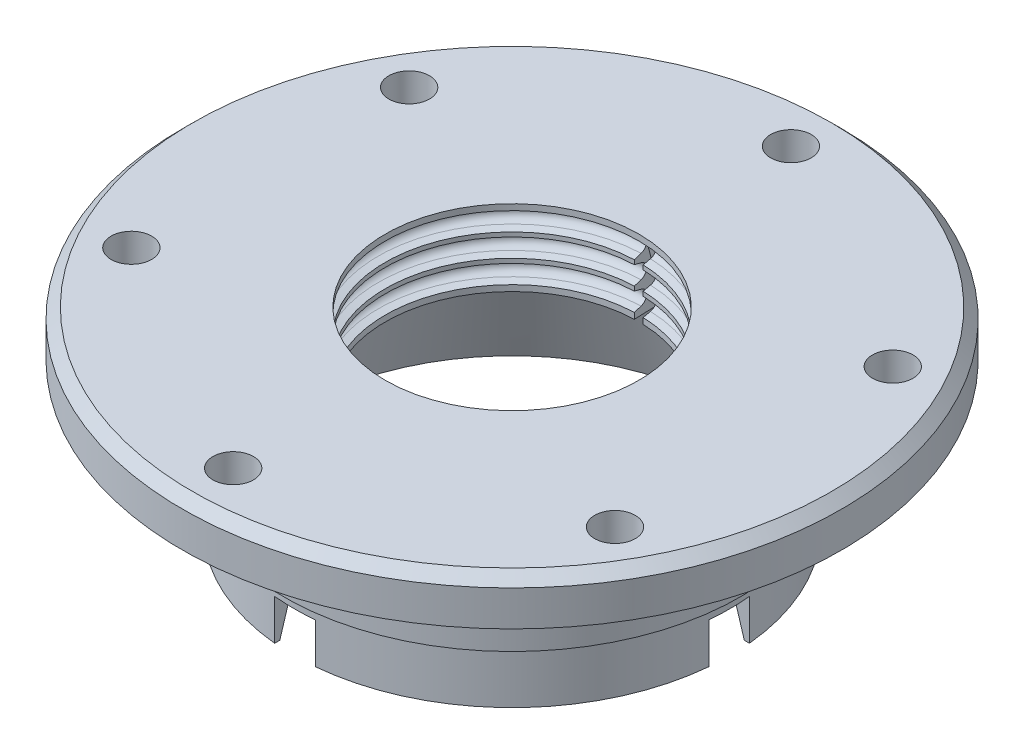
from build123d import *

# Parameters (mm, degrees)
FILLET1_R          = 5
SKETCH2_W          = 46.38448916527463
SKETCH2_H          = 8
CUT_EXTRUDE1_DEPTH = 4
SKETCH3_W          = 119.06569659747659
SKETCH3_H          = 8
CUT_EXTRUDE2_DEPTH = 4
CUT_REVOLVE2_ANGLE = 4.000000000000009
SKETCH5_R          = 3.999999999999999
SKETCH5_R_2        = 4.000000000000001
SKETCH5_R_3        = 4.000000000000005
CUT_EXTRUDE3_DEPTH = 94
SCALE_1_SCALE      = 1.875


with BuildPart() as part:
    # Sketch1 → Revolve1 (revolve)
    with BuildSketch(Plane.XY, mode=Mode.PRIVATE) as revolve1_sk:
        with BuildLine():
            Line((-43, -1.2e-16), (-43, 11))
            Line((-43, 11), (-45.00000000000001, 10.999999999999998))
            Line((-45.00000000000001, 10.999999999999998), (-45.00000000000001, 26.999999999999996))
            Line((-45.00000000000001, 26.999999999999996), (-43, 26.999999999999996))
            Line((-43, 26.999999999999996), (-43, 28.999999999999996))
            Line((-43, 28.999999999999996), (-65, 28.99999999999999))
            Line((-65, 28.99999999999999), (-65, 36))
            Line((-65, 36), (-63, 38))
            Line((-63, 38), (-25, 38))
            Line((-25, 38), (-25, 36.82086346304624))
            Line((-25, 36.82086346304624), (-26.388228567653783, 36.44888873943359))
            ThreePointArc((-26.388228567653783, 36.44888873943359), (-27.5, 34.99999999999999), (-26.388228567653783, 33.55111126056639))
            Line((-26.388228567653783, 33.55111126056639), (-25, 33.17913653695374))
            Line((-25, 33.17913653695374), (-25, 32.32086346304623))
            Line((-25, 32.32086346304623), (-26.38822856765378, 31.948888739433585))
            ThreePointArc((-26.38822856765378, 31.948888739433585), (-27.499999999999986, 30.5), (-26.388228567653783, 29.051111260566397))
            Line((-26.388228567653783, 29.051111260566397), (-25, 28.679136536953745))
            Line((-25, 28.679136536953745), (-25, 27.807055903779258))
            Line((-25, 27.807055903779258), (-26.57755901026072, 27.384350240967457))
            ThreePointArc((-26.57755901026072, 27.384350240967457), (-27.496662016431728, 25.899985958133367), (-26.38822856765378, 24.551111260566397))
            Line((-26.38822856765378, 24.551111260566397), (-25, 24.179136536953752))
            Line((-25, 24.179136536953752), (-24.999999999999996, 23))
            Line((-24.999999999999996, 23), (-34.99999999999999, 23))
            Line((-34.99999999999999, 23), (-42, 0))
            Line((-42, 0), (-43, -1.2e-16))
        make_face()
    revolve(revolve1_sk.sketch.rotate(Axis((0, 0, 0), (0, 1, 0)), 270), axis=Axis((0, 0, 0), (0, 1, 0)))

    # Fillet1
    fillet1_edges = [part.edges().sort_by_distance(p)[0] for p in [
        (-1.206e-14, 23, 34.99999999999999),
    ]]
    fillet(fillet1_edges, radius=FILLET1_R)

    # Sketch2 → Cut-Extrude1 (cut, symmetric)
    with BuildSketch(Plane.XY):
        with Locations((41.27123839114988, 4)):
            Rectangle(SKETCH2_W, SKETCH2_H)
        Polygon((-21.00085139372669, -1.2e-16), (-54.05436532646177, -1.2e-16), (-54.05436532646177, 7.9999999999999964), (-21.00085139372669, 8), align=None)
    extrude(amount=CUT_EXTRUDE1_DEPTH, both=True, mode=Mode.SUBTRACT)

    # Sketch3 → Cut-Extrude2 (cut, symmetric)
    with BuildSketch(Plane(origin=(0, 0, 0), x_dir=(0, 0, -1), z_dir=(1, 0, 0))):
        with Locations((-3.469705882441801, 4)):
            Rectangle(SKETCH3_W, SKETCH3_H)
    extrude(amount=CUT_EXTRUDE2_DEPTH, both=True, mode=Mode.SUBTRACT)

    # Sketch4 → Cut-Revolve2 (revolve, symmetric, cut)
    with BuildSketch(Plane(origin=(0, 0, 0), x_dir=(0, 0, -1), z_dir=(1, 0, 0))) as cut_revolve2_sk:
        with BuildLine():
            Line((-27.4488887394336, 35.38822856765377), (-30.768304579788595, 23))
            Line((-30.768304579788595, 23), (-24.499999999999996, 23))
            Line((-24.499999999999996, 23), (-24.499999999999996, 34.99999999999999))
            ThreePointArc((-24.499999999999996, 34.99999999999999), (-26.195789288330076, 33.51283270793928), (-27.4488887394336, 35.38822856765377))
        make_face()
        with BuildLine():
            Line((30.768304579788595, 23), (24.499999999999996, 23))
            Line((24.499999999999996, 23), (24.499999999999996, 34.99999999999999))
            ThreePointArc((24.499999999999996, 34.99999999999999), (26.195789288330076, 33.51283270793928), (27.4488887394336, 35.38822856765377))
            Line((27.4488887394336, 35.38822856765377), (30.768304579788595, 23))
        make_face()
    revolve(axis=Axis((0, 0, 0), (0, -1, 0)), revolution_arc=CUT_REVOLVE2_ANGLE / 2, mode=Mode.SUBTRACT)
    revolve(cut_revolve2_sk.sketch, axis=Axis((0, 0, 0), (0, 1, 0)), revolution_arc=CUT_REVOLVE2_ANGLE / 2, mode=Mode.SUBTRACT)

    # Sketch5 → Cut-Extrude3 (cut)
    with BuildSketch(Plane.XZ):
        with Locations(Location((-47.69194914270065, 27.394853293457416, 0), (0, 0, 270))):
            Circle(SKETCH5_R)
        with Locations(Location((0, 55, 0), (0, 0, 270))):
            Circle(SKETCH5_R_2)
        with Locations(Location((47.69194914270066, 27.394853293457416, 0), (0, 0, 270))):
            Circle(SKETCH5_R_3)
        with Locations(Location((-47.69194914270065, -27.394853293457416, 0), (0, 0, 270))):
            Circle(SKETCH5_R)
        with Locations(Location((0, -55, 0), (0, 0, 270))):
            Circle(SKETCH5_R_2)
        with Locations(Location((47.69194914270066, -27.394853293457416, 0), (0, 0, 270))):
            Circle(SKETCH5_R_3)
    extrude(amount=-CUT_EXTRUDE3_DEPTH, mode=Mode.SUBTRACT)


with BuildPart() as part_1:
    # Scale 1: scaled about (0, 28.362532631, 0)
    add(part.part.scale(SCALE_1_SCALE).moved(Location((0, -24.817216052125, 0))))


solid = part_1.part
